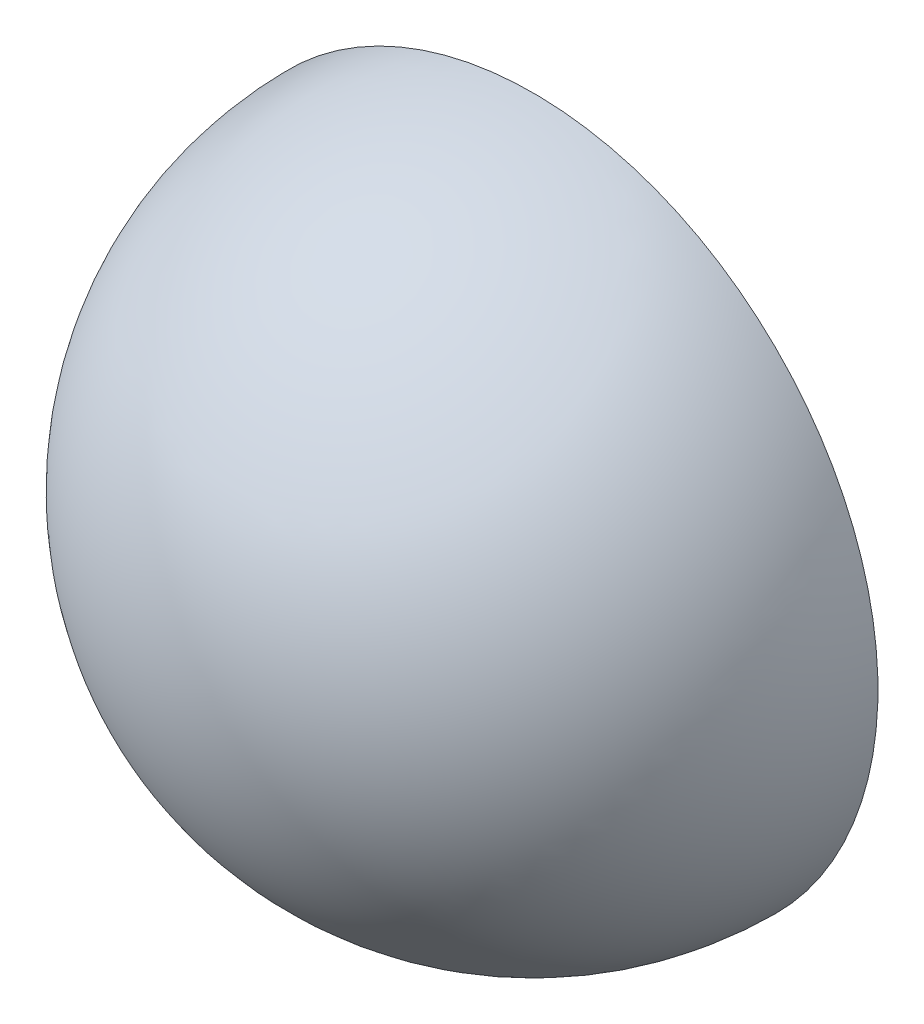
SolidWorks part; units mm, degrees
ref_plane "前视基准面" through (0, 0, 0) normal (0, 0, 1) x (1, 0, 0)
ref_plane "上视基准面" through (0, 0, 0) normal (0, 1, 0) x (1, 0, 0)
ref_plane "右视基准面" through (0, 0, 0) normal (1, 0, 0) x (0, 0, -1)
sketch "草图1" plane through (0, 0, 0) normal (0, 0, 1) x (1, 0, 0)
  line L0 (0, 70) -> (0, -70)
  arc A0 (0, -70) -> (0, 70) centre (0, 0) ccw
  dimension "D1" = 70
revolve "旋转1" add sketch "草图1" angle 180 about L0
